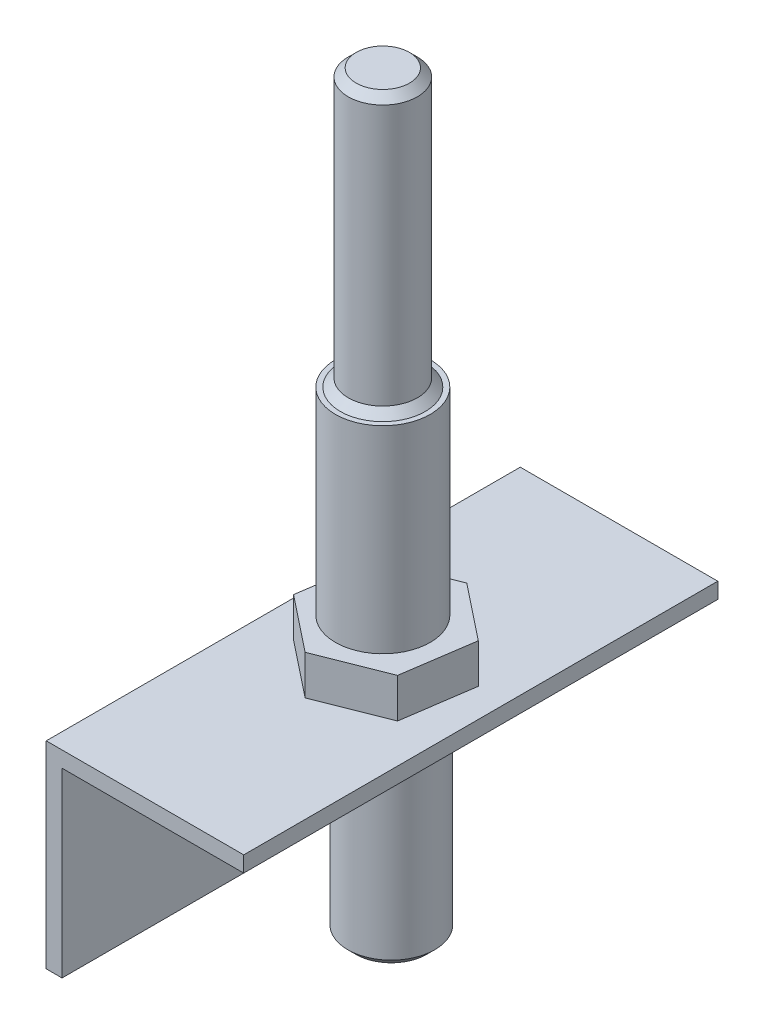
SolidWorks part; units mm, degrees
ref_plane "Front Plane" through (0, 0, 0) normal (0, 0, 1) x (1, 0, 0)
ref_plane "Top Plane" through (0, 0, 0) normal (0, 1, 0) x (1, 0, 0)
ref_plane "Right Plane" through (0, 0, 0) normal (1, 0, 0) x (0, 0, -1)
sketch "Sketch2" plane through (0, 0, 0) normal (0, 0, 1) x (1, 0, 0)
  line L0 (0, 0) -> (0, 25)
  line L1 (0, 25) -> (25, 25)
  dimension "D1" = 25
  dimension "D2" = 25
extrude "Extrude-Thin1" add sketch "Sketch2" along normal blind 60 thin
sketch "Sketch3" plane through (0, 25, 0) normal (0, 1, 0) x (1, 0, 0)
  line L0 (0, -60) -> (0, 0) construction
  line L1 (11.6849, -38.9111) -> (20.0597, -35.5944)
  line L2 (20.0597, -35.5944) -> (21.3748, -26.6833)
  line L3 (21.3748, -26.6833) -> (14.3151, -21.0889)
  line L4 (14.3151, -21.0889) -> (5.9403, -24.4056)
  line L5 (5.9403, -24.4056) -> (4.6252, -33.3167)
  line L6 (4.6252, -33.3167) -> (11.6849, -38.9111)
  circle A0 centre (13, -30) radius 7.8008 construction
  dimension "D1" = 13
extrude "Boss-Extrude2" add sketch "Sketch3" along normal mid plane 10
sketch "Sketch4" plane through (0, 20, 0) normal (0, -1, 0) x (-1, 0, 0)
  line L0 (-2, -60) -> (-2, 0) construction
  circle A0 centre (-13, -29.3194) radius 5.5
  dimension "D1" = 11
  dimension "D2" = 11
extrude "Boss-Extrude3" add sketch "Sketch4" along normal blind 25
sketch "Sketch5" plane through (0, 30, 0) normal (0, 1, 0) x (1, 0, 0)
  circle A0 centre (12.5192, -29.9151) radius 6
  dimension "D1" = 12
extrude "Boss-Extrude4" add sketch "Sketch5" along normal blind 25
sketch "Sketch6" plane through (0, 55, 0) normal (0, 1, 0) x (1, 0, 0)
  circle A0 centre (12.5192, -29.9151) radius 4.3725
extrude "Boss-Extrude5" add sketch "Sketch6" along normal blind 35
chamfer "Chamfer1" distance 1 angle 45 3 edges at (12.5192, 55, 34.2876) (13, -5, 23.8194) (12.5192, 90, 34.2876)
